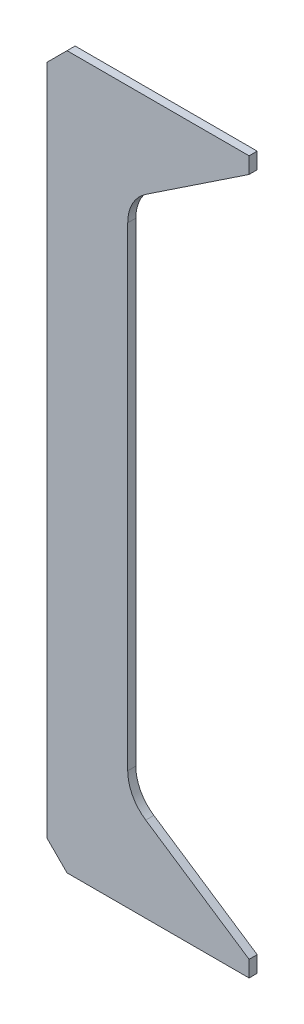
SolidWorks part; units mm, degrees
material "Q235B"
ref_plane "Front Plane" through (0, 0, 0) normal (0, 0, 1) x (1, 0, 0)
ref_plane "Top Plane" through (0, 0, 0) normal (0, 1, 0) x (1, 0, 0)
ref_plane "Right Plane" through (0, 0, 0) normal (1, 0, 0) x (0, 0, -1)
other "Configuration Table"
sketch "Sketch1" plane through (0, 0, 0) normal (0, 0, 1) x (1, 0, 0)
  line L0 (50, 0) -> (386.2279, 0) construction
  line L1 (-50, -440) -> (50, -440)
  line L2 (-50, -440) -> (-50, 440)
  line L3 (-50, 440) -> (50, 440)
  line L4 (50, -440) -> (50, 440)
  line L5 (-50, -440) -> (50, 440) construction
  line L6 (-50, 440) -> (50, -440) construction
  line L7 (-50, 440) -> (200, 440)
  line L8 (-50, 440) -> (-50, 420)
  line L9 (-50, 420) -> (200, 420)
  line L10 (200, 440) -> (200, 420)
  line L11 (200, 420) -> (50, 320)
  line L12 (200, -420) -> (50, -320)
  line L13 (200, -440) -> (200, -420)
  line L14 (-50, -420) -> (200, -420)
  line L15 (-50, -440) -> (-50, -420)
  line L16 (-50, -440) -> (200, -440)
  line L17 (-50, -440) -> (50, -440)
  point P0 (0, 0)
  dimension "D1" = 320
  dimension "D2" = 20
  dimension "D3" = 880
  dimension "D4" = 250
  dimension "D5" = 100
extrude "Boss-Extrude1" add sketch "Sketch1" along normal blind 10 contours L11 L9 L4 | L10 L7 L4 L9 | L2 L14 L4 L9 | L4 L14 L12 | L4 L16 L13 L14 | L14 L2 L1 L4 | L2 L9 L4 L3
fillet "Fillet1" radius 50 2 edges at (50, -320, 5) (50, 320, 5)
chamfer "Chamfer1" distance 25 angle 45 2 edges at (-50, 440, 5) (-50, -440, 5)
